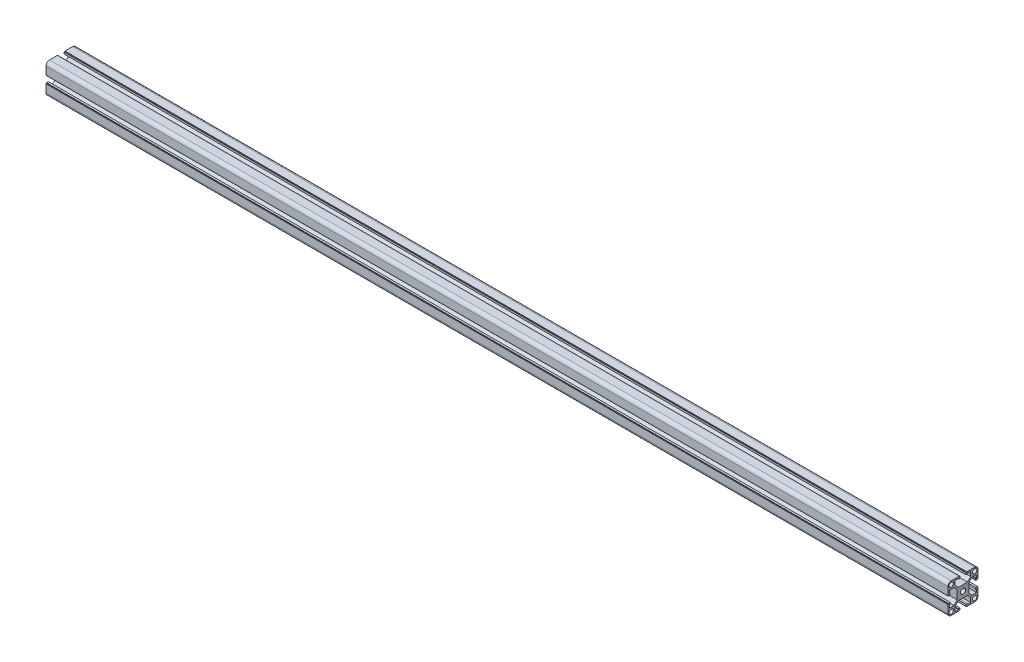
SolidWorks part; units mm, degrees
material "铝型材"
ref_plane "前基準面" through (0, 0, 0) normal (0, 0, 1) x (1, 0, 0)
ref_plane "上基準面" through (0, 0, 0) normal (0, 1, 0) x (1, 0, 0)
ref_plane "右基準面" through (0, 0, 0) normal (1, 0, 0) x (0, 0, -1)
sketch "草图1" plane through (0, 0, 0) normal (0, 1, 0) x (1, 0, 0)
  line L0 (-600, 0) -> (600, 0)
  dimension "D1" = 1200
other "铝型材 40 X 40W X R4.5(1)"
ref_plane "基准面1" through (-600, 0, 0) normal (1, 0, 0) x (0, 0, -1)
sketch "Sketch1" plane through (-600, 0, 0) normal (1, 0, 0) x (0, 0, -1)
  line L0 (-5.1, 20) -> (-5.1, 19.5)
  line L1 (-5.1, 19.5) -> (-4.1, 19.5)
  line L2 (-4.1, 19.5) -> (-4.1, 17)
  line L3 (-6.1, 18) -> (-10.3, 18)
  line L4 (-15.5, -20) -> (-5.1, -20)
  line L5 (-20, -15.5) -> (-20, -5.1)
  line L6 (15.5, 20) -> (5.1, 20)
  line L7 (20, 15.5) -> (20, 5.1)
  line L8 (0, 20) -> (0, 0) construction
  line L9 (0, 0) -> (20, 0) construction
  line L10 (-10.3, 18) -> (-10.3, 12)
  line L11 (-10.3, 12) -> (-6, 7.7)
  line L12 (-6, 7.7) -> (6, 7.7)
  line L13 (10.3, 12) -> (6, 7.7)
  line L14 (10.3, 18) -> (10.3, 12)
  line L15 (6.1, 18) -> (10.3, 18)
  line L16 (4.1, 19.5) -> (4.1, 17)
  line L17 (5.1, 19.5) -> (4.1, 19.5)
  line L18 (5.1, 20) -> (5.1, 19.5)
  line L19 (-5.1, 20) -> (-15.5, 20)
  line L20 (20, 5.1) -> (19.5, 5.1)
  line L21 (0, 0) -> (-15.5563, 15.5563) construction
  line L22 (0, 0) -> (-15.5563, -15.5563) construction
  line L23 (0, 20) -> (0, 40) construction
  line L24 (20, 0) -> (40, 0) construction
  line L25 (19.5, 5.1) -> (19.5, 4.1)
  line L26 (19.5, 4.1) -> (17, 4.1)
  line L27 (17, 6.1) -> (17, 4.1)
  line L28 (18, 6.1) -> (17, 6.1)
  line L29 (18, 6.1) -> (18, 10.3)
  line L30 (18, 10.3) -> (12, 10.3)
  line L31 (12, 10.3) -> (7.7, 6)
  line L32 (7.7, 6) -> (7.7, -6)
  line L33 (12, -10.3) -> (7.7, -6)
  line L34 (18, -10.3) -> (12, -10.3)
  line L35 (18, -6.1) -> (18, -10.3)
  line L36 (18, -6.1) -> (17, -6.1)
  line L37 (17, -4.1) -> (17, -6.1)
  line L38 (19.5, -4.1) -> (17, -4.1)
  line L39 (19.5, -5.1) -> (19.5, -4.1)
  line L40 (20, -5.1) -> (19.5, -5.1)
  line L41 (5.1, -20) -> (5.1, -19.5)
  line L42 (5.1, -19.5) -> (4.1, -19.5)
  line L43 (4.1, -19.5) -> (4.1, -17)
  line L44 (6.1, -17) -> (4.1, -17)
  line L45 (6.1, -18) -> (6.1, -17)
  line L46 (6.1, -18) -> (10.3, -18)
  line L47 (10.3, -18) -> (10.3, -12)
  line L48 (10.3, -12) -> (6, -7.7)
  line L49 (6, -7.7) -> (-6, -7.7)
  line L50 (-10.3, -12) -> (-6, -7.7)
  line L51 (-10.3, -18) -> (-10.3, -12)
  line L52 (-6.1, -18) -> (-10.3, -18)
  line L53 (-6.1, -18) -> (-6.1, -17)
  line L54 (-4.1, -17) -> (-6.1, -17)
  line L55 (-4.1, -19.5) -> (-4.1, -17)
  line L56 (-5.1, -19.5) -> (-4.1, -19.5)
  line L57 (-5.1, -20) -> (-5.1, -19.5)
  line L58 (-20, -5.1) -> (-19.5, -5.1)
  line L59 (5.1, -20) -> (15.5, -20)
  line L60 (-20, 5.1) -> (-20, 15.5)
  line L61 (-19.5, -5.1) -> (-19.5, -4.1)
  line L62 (-6.1, 18) -> (-6.1, 17)
  line L63 (-6.1, 17) -> (-4.1, 17)
  line L64 (6.1, 18) -> (6.1, 17)
  line L65 (4.1, 17) -> (6.1, 17)
  line L66 (-19.5, -4.1) -> (-17, -4.1)
  line L71 (-17, -6.1) -> (-17, -4.1)
  line L72 (-18, -6.1) -> (-17, -6.1)
  line L73 (-18, -6.1) -> (-18, -10.3)
  line L74 (-18, -10.3) -> (-12, -10.3)
  line L75 (-12, -10.3) -> (-7.7, -6)
  line L76 (-7.7, -6) -> (-7.7, 6)
  line L77 (-12, 10.3) -> (-7.7, 6)
  line L78 (-18, 10.3) -> (-12, 10.3)
  line L79 (-18, 6.1) -> (-18, 10.3)
  line L80 (-18, 6.1) -> (-17, 6.1)
  line L81 (-17, 4.1) -> (-17, 6.1)
  line L82 (-19.5, 4.1) -> (-17, 4.1)
  line L83 (-19.5, 5.1) -> (-19.5, 4.1)
  line L84 (-20, 5.1) -> (-19.5, 5.1)
  line L85 (20, -5.1) -> (20, -15.5)
  circle A0 centre (0, 0) radius 3.4
  arc A1 (-20, 15.5) -> (-15.5, 20) centre (-15.5, 15.5) cw
  arc A2 (20, 15.5) -> (15.5, 20) centre (15.5, 15.5) ccw
  arc A3 (-15.5, -20) -> (-20, -15.5) centre (-15.5, -15.5) cw
  arc A4 (15.5, -20) -> (20, -15.5) centre (15.5, -15.5) ccw
  circle A5 centre (-15.5563, 15.5563) radius 3
  circle A6 centre (15.5563, 15.5563) radius 3
  circle A7 centre (15.5563, -15.5563) radius 3
  circle A8 centre (-15.5563, -15.5563) radius 3
  point P2 (0, 10)
  point P4 (0, 0)
  point P5 (-20, -20)
  point P6 (20, -20)
  point P7 (20, 20)
  point P8 (-20, 20)
  point P13 (20, 0)
  point P36 (-20, 20)
  point P39 (20, 20)
  point P43 (0, 20)
  point P50 (-40, 0)
  point P59 (0, 40)
  point P72 (40, 0)
  point P73 (-20, 0)
  point P86 (10, 0)
  point P87 (-10, 0)
  point P88 (0, -10)
  point P89 (0, -20)
  point P117 (0, -40)
  point P118 (0, 0)
  dimension "D1" = 20.6
  dimension "D2" = 40
  dimension "D3" = 8.2
  dimension "D4" = 10.2
  dimension "D5" = 12.3
  dimension "D6" = 6.8
  dimension "D7" = 4.5
  dimension "D8" = 45
  dimension "D12" = 6
  dimension "D13" = 22
  dimension "D9" = 0.5
  dimension "D10" = 2
  dimension "D11" = 12
  dimension "D16" = 3
  dimension "D17" = 2
